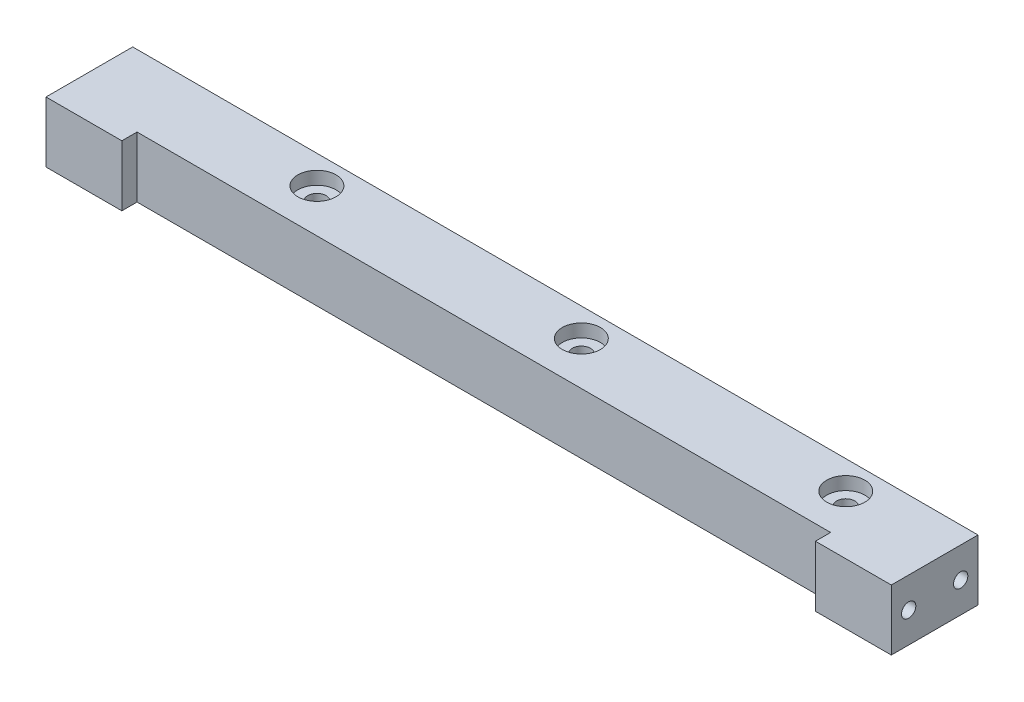
SolidWorks part; units mm, degrees
ref_plane "Front Plane" through (0, 0, 0) normal (0, 0, 1) x (1, 0, 0)
ref_plane "Top Plane" through (0, 0, 0) normal (0, 1, 0) x (1, 0, 0)
ref_plane "Right Plane" through (0, 0, 0) normal (1, 0, 0) x (0, 0, -1)
sketch "Sketch1" plane through (0, 0, 0) normal (0, 0, 1) x (1, 0, 0)
  line L1 (0, 0) -> (-195, 0)
  dimension "D2" = 195
extrude "Extrude-Thin1" add sketch "Sketch1" along normal mid plane 20 thin
hole_wizard "M4 Tapped Hole1" positions "Sketch2" profile "Sketch3" tap size "M4" standard "ISO"
sketch "Sketch2" plane through (-195, 0, 0) normal (-1, 0, 0) x (0, 0, 1)
  line L0 (0, 0) -> (0, -5.1315) construction
  line L1 (10, 0) -> (-10, 0) construction
  line L3 (-10, 7) -> (-6, 7) construction
  line L4 (-10, 0) -> (-10, 14) construction
  point P0 (-6, 7)
  point P2 (6, 7)
  dimension "D1" = 12
sketch "Sketch3" plane through (-195, 7, -6) normal (0, 1, 0) x (0, 0, 1)
  line L0 (0, 0) -> (0, 11.0914)
  line L1 (0, 11.0914) -> (1.65, 10.1)
  line L2 (1.65, 10.1) -> (1.65, 0)
  line L5 (1.65, 0) -> (0, 0)
  line L10 (0, 11.0914) -> (-1.65, 10.1) construction
  line L11 (0, -6.35) -> (0, 107.95) construction
  dimension "螺纹孔钻头直径" = 3.3
  dimension "螺纹孔钻头深度" = 10.1
  dimension "导头角度" = 118
cosmetic thread "Cosmetic Thread1" parameters "D1"=8, "D2"=4
cosmetic thread "Cosmetic Thread2" parameters "D1"=8, "D2"=4
hole_wizard "M4 Tapped Hole2" positions "Sketch4" profile "Sketch5" tap size "M4" standard "ISO"
sketch "Sketch4" plane through (0, 0, 0) normal (1, 0, 0) x (0, 0, -1)
  point P0 (-6, 7)
  point P3 (6, 7)
sketch "Sketch5" plane through (0, 7, 6) normal (0, 1, 0) x (0, 0, -1)
  line L0 (0, 0) -> (0, 11.0914)
  line L1 (0, 11.0914) -> (1.65, 10.1)
  line L2 (1.65, 10.1) -> (1.65, 0)
  line L5 (1.65, 0) -> (0, 0)
  line L10 (0, 11.0914) -> (-1.65, 10.1) construction
  line L11 (0, -6.35) -> (0, 107.95) construction
  dimension "螺纹孔钻头直径" = 3.3
  dimension "螺纹孔钻头深度" = 10.1
  dimension "导头角度" = 118
cosmetic thread "Cosmetic Thread3" parameters "D1"=8, "D2"=4
cosmetic thread "Cosmetic Thread4" parameters "D1"=8, "D2"=4
hole_wizard "M5 Tapped Hole1" positions "Sketch6" profile "Sketch8" tap size "M5" standard "ISO" end condition through all
sketch "Sketch6" plane through (0, 14, 0) normal (0, 1, 0) x (1, 0, 0)
  line L1 (-195, -10) -> (-195, 10) construction
  line L2 (0, 10) -> (-195, 10) construction
  point P0 (-146, 3.5)
  point P2 (-85, 3.5)
  point P4 (-24, 3.5)
  dimension "D1" = 6.5
  dimension "D2" = 49
  dimension "D3" = 61
  dimension "D4" = 61
sketch "Sketch8" plane through (-146, 14, -3.5) normal (1, 0, 0) x (0, 0, 1)
  line L0 (0, 0) -> (0, 14)
  line L1 (0, 14) -> (2.1, 14)
  line L2 (2.1, 14) -> (2.1, 0)
  line L5 (2.1, 0) -> (0, 0)
  line L11 (0, -6.35) -> (0, 107.95) construction
  dimension "通孔螺纹孔钻头直径" = 4.2
  dimension "通孔螺纹孔钻头深度" = 14
cosmetic thread "Cosmetic Thread5" parameters "D2"=5
cosmetic thread "Cosmetic Thread6" parameters "D2"=5
cosmetic thread "Cosmetic Thread7" parameters "D2"=5
sketch "Sketch9" plane through (0, 14, 0) normal (0, 1, 0) x (1, 0, 0)
  circle A0 centre (-146, 3.5) radius 4.4
  circle A1 centre (-85, 3.5) radius 4.4
  circle A2 centre (-24, 3.5) radius 4.4
  dimension "D1" = 8.8
extrude "Cut-Extrude1" cut sketch "Sketch9" against normal blind 3
sketch "Sketch10" plane through (0, 14, 0) normal (0, 1, 0) x (1, 0, 0)
  line L0 (0, -10) -> (-195, -10) construction
  line L1 (-177.5, -10) -> (-17.5, -10)
  line L2 (-177.5, -10) -> (-177.5, -6.5)
  line L3 (-177.5, -6.5) -> (-17.5, -6.5)
  line L4 (-17.5, -10) -> (-17.5, -6.5)
  line L5 (-97.5, 10) -> (-97.5, -6.5) construction
  line L6 (0, 10) -> (-195, 10) construction
  dimension "D1" = 3.5
  dimension "D2" = 160
extrude "Cut-Extrude2" cut sketch "Sketch10" against normal blind 20
